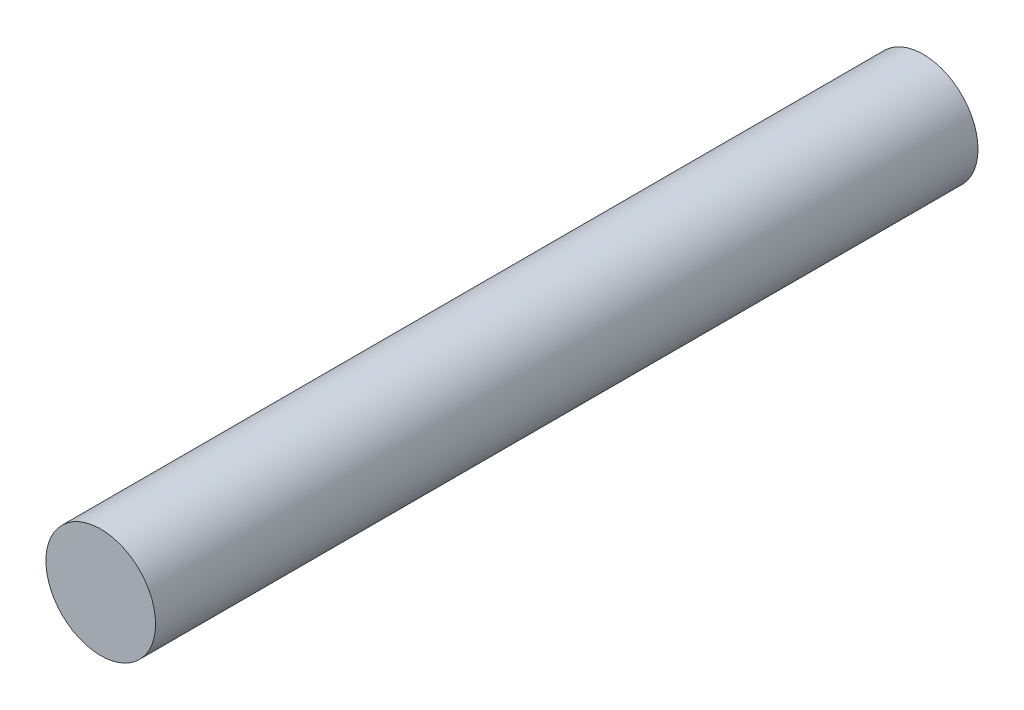
from build123d import *

# Parameters (mm, degrees)
SKETCH_1_R      = 10
EXTRUDE_1_DEPTH = 75


with BuildPart() as part:
    # 草图1 → 凸台-拉伸1 (new, symmetric)
    with BuildSketch(Plane.XY):
        Circle(SKETCH_1_R)
    extrude(amount=EXTRUDE_1_DEPTH, both=True)


solid = part.part
